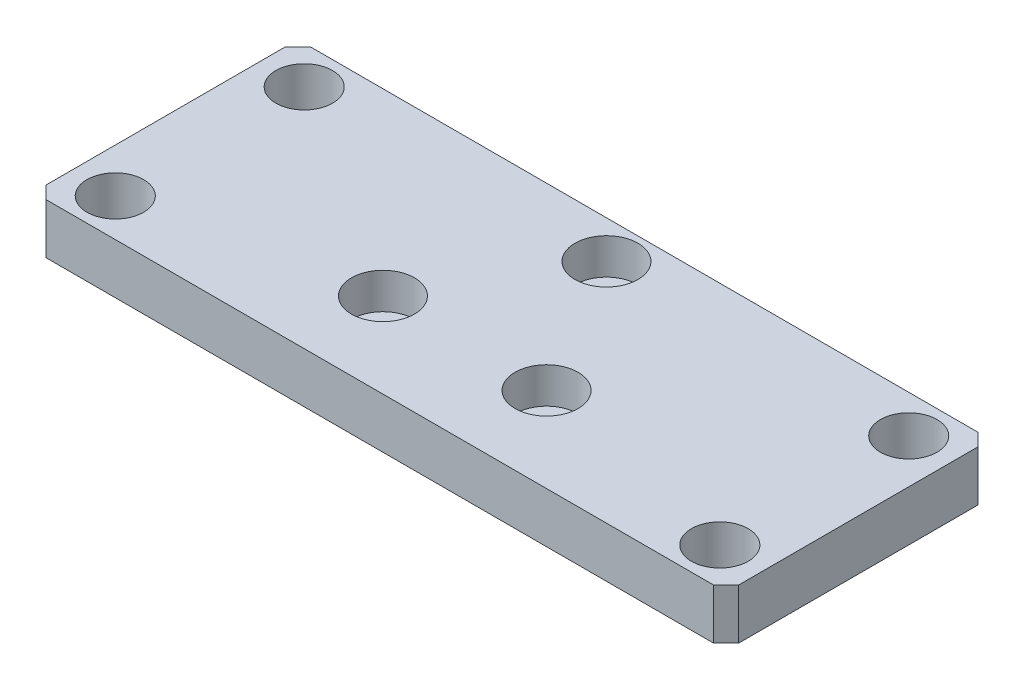
SolidWorks part; units mm, degrees
ref_plane "前视基准面" through (0, 0, 0) normal (0, 0, 1) x (1, 0, 0)
ref_plane "上视基准面" through (0, 0, 0) normal (0, 1, 0) x (1, 0, 0)
ref_plane "右视基准面" through (0, 0, 0) normal (1, 0, 0) x (0, 0, -1)
sketch "草图1" plane through (0, 0, 0) normal (0, 1, 0) x (1, 0, 0)
  line L1 (-55, 21) -> (55, 21)
  line L2 (-55, 21) -> (-55, -21)
  line L3 (-55, -21) -> (55, -21)
  line L4 (55, 21) -> (55, -21)
  line L5 (-55, 21) -> (55, -21) construction
  line L6 (-55, -21) -> (55, 21) construction
  point P0 (0, 0)
  dimension "D1" = 110
  dimension "D2" = 42
extrude "凸台-拉伸1" add sketch "草图1" along normal mid plane 8
hole_wizard "M6 六角凹头螺钉的柱形沉头孔1" positions "草图6" profile "草图4" counterbore size "M6" standard "ISO" end condition through all
sketch "草图6" plane through (0, 4, 0) normal (0, 1, 0) x (1, 0, 0)
  line L1 (0, 0) -> (0, 23.1773) construction
  line L7 (0, 0) -> (-20.1366, -11.6259) construction
  line L9 (0, 0) -> (18.0246, -10.4065) construction
  circle A0 centre (0, 0) radius 15 construction
  point P0 (0, 15)
  point P2 (-12.9904, -7.5)
  point P4 (12.9904, -7.5)
  dimension "D1" = 30
  dimension "D2" = 120
  dimension "D3" = 120
sketch "草图4" plane through (0, 4, -15) normal (1, 0, 0) x (0, 0, 1)
  line L0 (0, 0) -> (0, 8)
  line L1 (0, 8) -> (2.75, 8)
  line L3 (2.75, 8) -> (2.75, 5.7)
  line L4 (2.75, 5.7) -> (5, 5.7)
  line L5 (5, 5.7) -> (5, 0)
  line L7 (5, 0) -> (0, 0)
  line L11 (0, -6.35) -> (0, 107.95) construction
  dimension "通孔孔直径" = 5.5
  dimension "通孔孔深度" = 8
  dimension "柱形沉头孔直径" = 10
  dimension "柱形沉头孔深度" = 5.7
hole_wizard "Ø9.0 (9) 直径孔1" positions "草图8" profile "草图7" hole size "Ø9.0" standard "ISO" end condition through all
sketch "草图8" plane through (0, -4, 0) normal (0, -1, 0) x (-1, 0, 0)
  line L1 (0, 0) -> (-57.0854, 0) construction
  point P0 (-48, -15)
  dimension "D1" = 15
  dimension "D2" = 48
sketch "草图7" plane through (48, -4, 15) normal (1, 0, 0) x (0, 0, -1)
  line L0 (0, 0) -> (0, 8)
  line L1 (0, 8) -> (4.5, 8)
  line L2 (4.5, 8) -> (4.5, 0)
  line L5 (4.5, 0) -> (0, 0)
  line L11 (0, -6.35) -> (0, 107.95) construction
  dimension "通孔孔直径" = 9
  dimension "通孔孔深度" = 8
chamfer "倒角1" distance 2 angle 45 4 edges at (-55, 0, 21) (55, 0, 21) (55, 0, -21) (-55, 0, -21)
mirror "镜向1" about plane through (0, 0, 0) normal (0, 0, 1) of "Ø9.0 (9) 直径孔1"
mirror "镜向2" about plane through (0, 0, 0) normal (1, 0, 0) of "镜向1", "Ø9.0 (9) 直径孔1"
